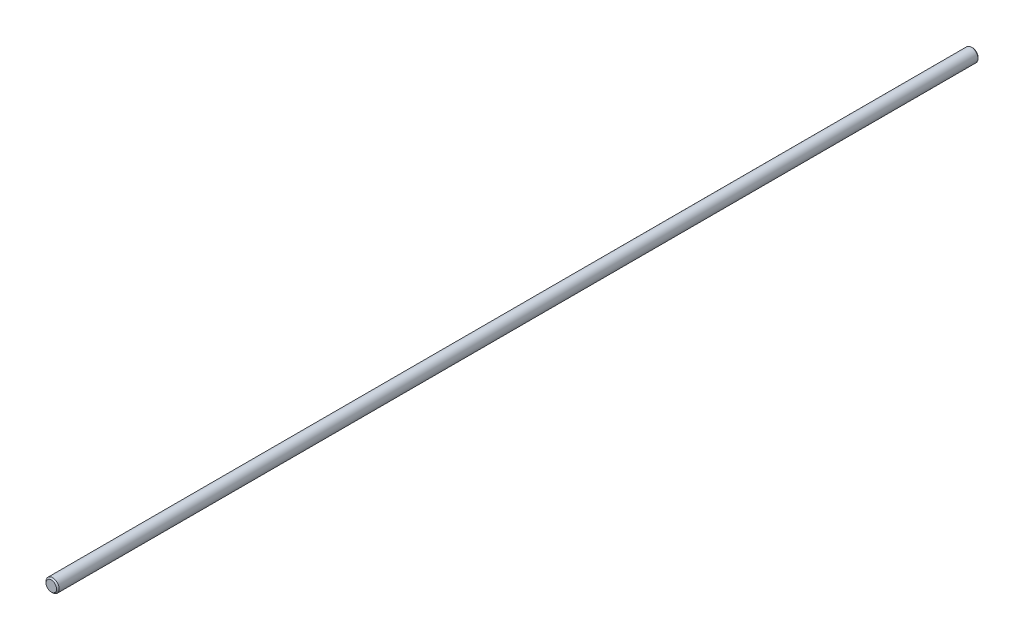
SolidWorks part; units mm, degrees
ref_plane "Front Plane" through (0, 0, 0) normal (0, 0, 1) x (1, 0, 0)
ref_plane "Top Plane" through (0, 0, 0) normal (0, 1, 0) x (1, 0, 0)
ref_plane "Right Plane" through (0, 0, 0) normal (1, 0, 0) x (0, 0, -1)
sketch "Sketch1" plane through (0, 0, 0) normal (0, 0, 1) x (1, 0, 0)
  circle A0 centre (0, 0) radius 5
  dimension "D1" = 10
extrude "Boss-Extrude1" add sketch "Sketch1" along normal mid plane 700
cosmetic thread "Cosmetic Thread1" parameters "D1"=25, "D2"=8.344
cosmetic thread "Cosmetic Thread2" parameters "D1"=25, "D2"=8.344
chamfer "Chamfer1" distance 1 angle 45 2 edges at (5, 0, 350) (5, 0, -350)
